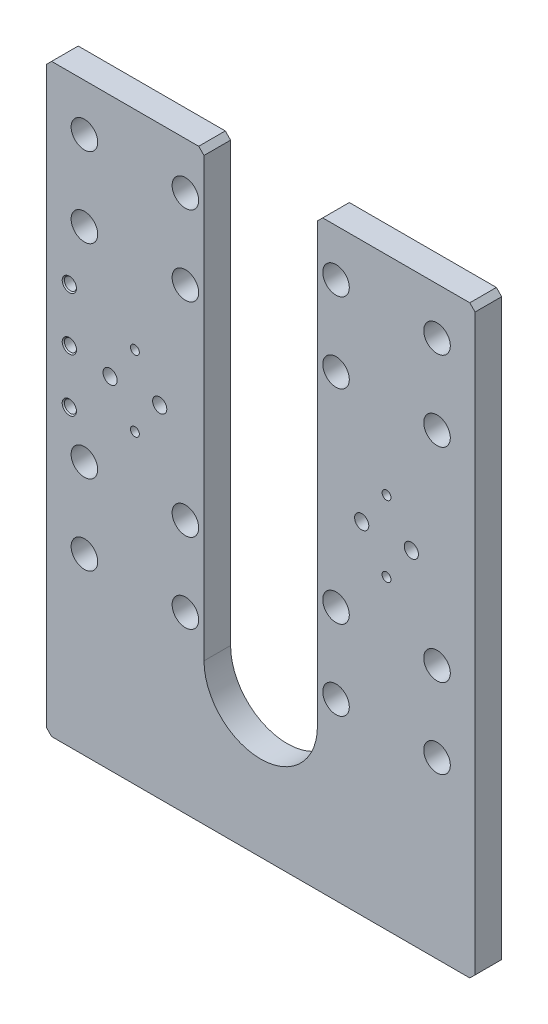
from build123d import *

# Parameters (mm, degrees)
BOSS_EXTRUDE1_DEPTH         = 15
CHAMFER1_SIZE               = 3
HOLE1_D                     = 9
HOLE1_CBORE_D               = 15
HOLE1_CBORE_DEPTH           = 10.6
M8_TAPPED_HOLE1_D           = 6.8
M8_TAPPED_HOLE1_CSINK_D     = 8.05
M8_TAPPED_HOLE1_CSINK_ANGLE = 90
HOLE2_D                     = 8
HOLE2_DEPTH                 = 8
M6_TAPPED_HOLE1_D           = 5


with BuildPart() as part:
    # Sketch1 → Boss-Extrude1 (new body)
    with BuildSketch(Plane.XY):
        with BuildLine():
            Line((-117.978782331, 156.590116279), (-28.978782331, 156.590116279))
            Line((-28.978782331, 156.590116279), (-28.978782331, -93.409883721))
            ThreePointArc((-28.978782331, -93.409883721), (3.021217669, -125.409883721), (35.021217669, -93.409883721))
            Line((35.021217669, -93.409883721), (35.021217669, 156.590116279))
            Line((35.021217669, 156.590116279), (124.021217669, 156.590116279))
            Line((124.021217669, 156.590116279), (124.021217669, -173.409883721))
            Line((124.021217669, -173.409883721), (-117.978782331, -173.409883721))
            Line((-117.978782331, -173.409883721), (-117.978782331, 156.590116279))
        make_face()
    extrude(amount=BOSS_EXTRUDE1_DEPTH)

    # Chamfer1
    chamfer1_edges = [part.edges().sort_by_distance(p)[0] for p in [
        (-117.978782331, 156.590116279, 7.5),
        (-28.978782331, 156.590116279, 7.5),
        (35.021217669, 156.590116279, 7.5),
        (124.021217669, 156.590116279, 7.5),
        (124.021217669, -173.409883721, 7.5),
        (-117.978782331, -173.409883721, 7.5),
    ]]
    chamfer(chamfer1_edges, length=CHAMFER1_SIZE)

    # Hole1 (through all)
    with Locations(Plane.XY.offset(15)):
        with Locations((-96.478782331, 130.052169647), (-39.478782331, 130.052169647), (-39.478782331, 85.052169647), (-96.478782331, 85.052169647), (-96.478782331, -29.947830353), (-39.478782331, -29.947830353), (-39.478782331, -74.947830353), (-96.478782331, -74.947830353), (45.521217669, -74.947830353), (45.521217669, -29.947830353), (102.521217669, -29.947830353), (102.521217669, -74.947830353), (45.521217669, 85.052169647), (45.521217669, 130.052169647), (102.521217669, 130.052169647), (102.521217669, 85.052169647)):
            CounterBoreHole(HOLE1_D / 2, HOLE1_CBORE_D / 2, HOLE1_CBORE_DEPTH)

    # M8 Tapped Hole1 (through all)
    with Locations(Plane.XY.offset(15)):
        with Locations((-104.978782331, 52.590116279), (-104.978782331, 22.590116279), (-104.978782331, -7.409883721)):
            CounterSinkHole(M8_TAPPED_HOLE1_D / 2, M8_TAPPED_HOLE1_CSINK_D / 2, counter_sink_angle=M8_TAPPED_HOLE1_CSINK_ANGLE)

    # Hole2
    with Locations(Plane.XY.offset(15)):
        with Locations((-81.978782331, 19.090116279), (-53.978782331, 19.090116279), (60.021217669, 19.090116279), (88.021217669, 19.090116279)):
            Hole(HOLE2_D / 2, depth=HOLE2_DEPTH)

    # M6 Tapped Hole1 (through all)
    with Locations(Plane(origin=(0, 0, 0), x_dir=(-1, 0, 0), z_dir=(0, 0, -1))):
        with Locations((-74.021217669, 39.090116279), (-74.021217669, -0.909883721), (67.978782331, -0.909883721), (67.978782331, 39.090116279)):
            Hole(M6_TAPPED_HOLE1_D / 2)


solid = part.part
